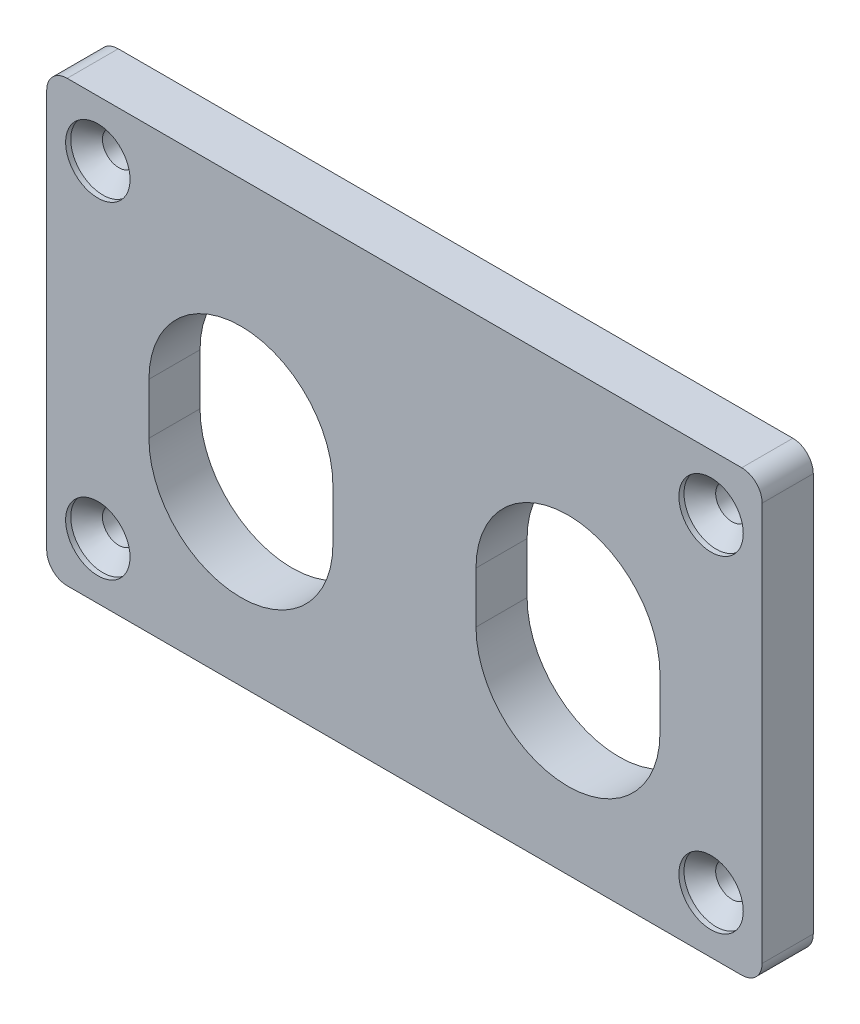
SolidWorks part; units mm, degrees
ref_plane "Front Plane" through (0, 0, 0) normal (0, 0, 1) x (1, 0, 0)
ref_plane "Top Plane" through (0, 0, 0) normal (0, 1, 0) x (1, 0, 0)
ref_plane "Right Plane" through (0, 0, 0) normal (1, 0, 0) x (0, 0, -1)
sketch "Sketch1" plane through (0, 0, 0) normal (0, 0, 1) x (1, 0, 0)
  line L0 (19, 21.5) -> (19, 16.5) construction
  line L1 (2, 0) -> (68, 0)
  line L2 (0, 2) -> (0, 41)
  line L3 (2, 43) -> (68, 43)
  line L4 (70, 2) -> (70, 41)
  line L5 (28, 21.5) -> (28, 16.5)
  line L6 (10, 21.5) -> (10, 16.5)
  line L7 (51, 21.5) -> (51, 16.5) construction
  line L8 (60, 21.5) -> (60, 16.5)
  line L9 (42, 21.5) -> (42, 16.5)
  line L10 (35, 43) -> (35, 0) construction
  arc A0 (68, 43) -> (70, 41) centre (68, 41) cw
  arc A1 (68, 0) -> (70, 2) centre (68, 2) ccw
  arc A2 (2, 0) -> (0, 2) centre (2, 2) cw
  arc A3 (0, 41) -> (2, 43) centre (2, 41) cw
  arc A4 (28, 21.5) -> (10, 21.5) centre (19, 21.5) ccw
  arc A5 (10, 16.5) -> (28, 16.5) centre (19, 16.5) ccw
  arc A6 (60, 21.5) -> (42, 21.5) centre (51, 21.5) ccw
  arc A7 (42, 16.5) -> (60, 16.5) centre (51, 16.5) ccw
  point P9 (70, 0)
  point P12 (0, 0)
  point P15 (0, 43)
  point P18 (19, 19)
  point P23 (51, 19)
  dimension "D3" = 2
  dimension "D4" = 9
  dimension "D1" = 43
  dimension "D2" = 70
  dimension "D5" = 5
  dimension "D6" = 19
  dimension "D7" = 32
extrude "Boss-Extrude1" add sketch "Sketch1" along normal blind 5
hole_wizard "CSK for M3 Flat Head Machine Screw1" positions "Sketch3" profile "Sketch2" countersink size "M3" standard "Ansi Metric" end condition through all
sketch "Sketch3" plane through (0, 0, 5) normal (0, 0, 1) x (1, 0, 0)
  line L0 (0, 21.5) -> (70, 21.5) construction
  line L1 (0, 41) -> (0, 2) construction
  line L2 (70, 2) -> (70, 41) construction
  line L4 (35, 43) -> (35, 0) construction
  line L5 (68, 43) -> (2, 43) construction
  line L6 (2, 0) -> (68, 0) construction
  point P0 (5, 37.5)
  point P1 (5, 5.5)
  point P3 (65, 5.5)
  point P5 (65, 37.5)
  dimension "D1" = 60
  dimension "D2" = 32
sketch "Sketch2" plane through (5, 37.5, 5) normal (1, 0, 0) x (0, -1, 0)
  line L0 (0, 0) -> (0, 5)
  line L1 (0, 5) -> (1.6, 5)
  line L2 (1.6, 5) -> (1.6, 2.05)
  line L3 (1.6, 2.05) -> (3.15, 0.5)
  line L4 (3.15, 0.5) -> (3.15, 0)
  line L6 (3.15, 0) -> (0, 0)
  line L7 (-1.6, 2.05) -> (-3.15, 0.5) construction
  line L11 (0, -6.35) -> (0, 107.95) construction
  dimension "通孔孔直径" = 3.2
  dimension "通孔孔深度" = 5
  dimension "锥形沉头孔直径" = 6.3
  dimension "锥形沉头孔角度" = 90
  dimension "头间隙" = 0.5
